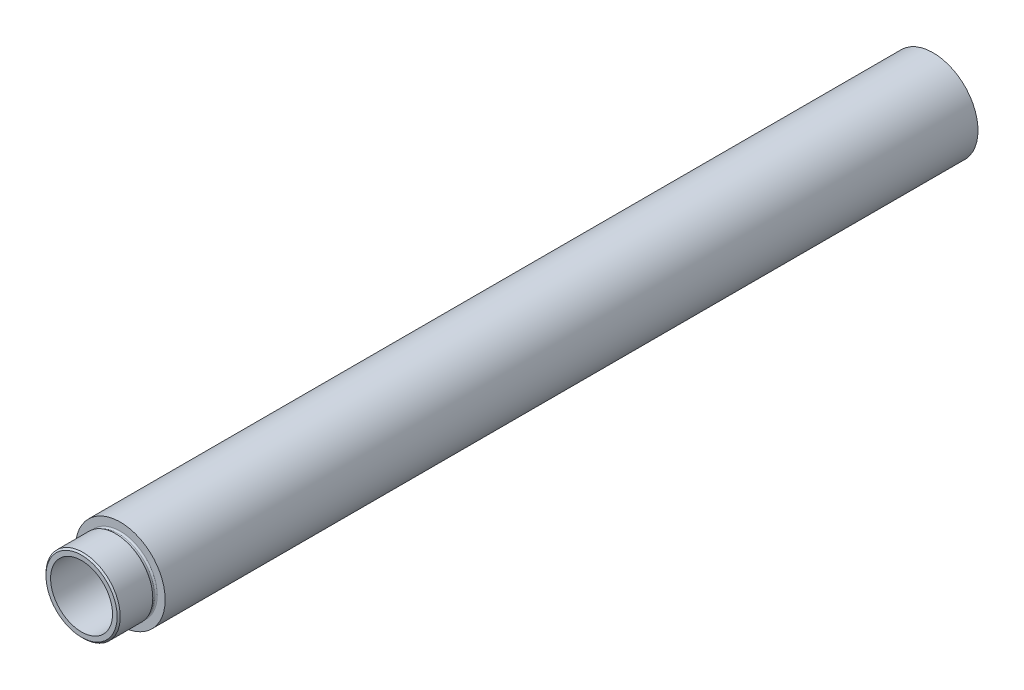
from build123d import *

# Parameters (mm, degrees)
SKETCH1_R           = 29
BOSS_EXTRUDE1_DEPTH = 550
CUT_EXTRUDE1_START  = -25
SKETCH2_R           = 29
SKETCH2_R_2         = 24
CUT_EXTRUDE1_DEPTH  = 25
SKETCH3_R           = 20
CUT_EXTRUDE2_DEPTH  = 552.526971235
CHAMFER1_SIZE       = 1
SKETCH4_R           = 24
SKETCH4_R_2         = 22.9
CUT_EXTRUDE3_DEPTH  = 3
FILLET1_R           = 1


with BuildPart() as part:
    # Sketch1 → Boss-Extrude1 (new body)
    with BuildSketch(Plane.XY):
        Circle(SKETCH1_R)
    extrude(amount=BOSS_EXTRUDE1_DEPTH)

    # Sketch2 → Cut-Extrude1 (cut)
    with BuildSketch(Plane.XY.offset(550).offset(CUT_EXTRUDE1_START)):
        Circle(SKETCH2_R)
        Circle(SKETCH2_R_2, mode=Mode.SUBTRACT)
    extrude(amount=CUT_EXTRUDE1_DEPTH, mode=Mode.SUBTRACT)

    # Sketch3 → Cut-Extrude2 (cut, through all)
    with BuildSketch(Plane.XY.offset(550)):
        Circle(SKETCH3_R)
    extrude(amount=-CUT_EXTRUDE2_DEPTH, mode=Mode.SUBTRACT)

    # Chamfer1
    chamfer1_edges = [part.edges().sort_by_distance(p)[0] for p in [
        (-24, 0, 550),
    ]]
    chamfer(chamfer1_edges, length=CHAMFER1_SIZE)

    # Sketch4 → Cut-Extrude3 (cut)
    with BuildSketch(Plane.XY.offset(525)):
        Circle(SKETCH4_R)
        Circle(SKETCH4_R_2, mode=Mode.SUBTRACT)
    extrude(amount=CUT_EXTRUDE3_DEPTH, mode=Mode.SUBTRACT)

    # Fillet1
    fillet1_edges = [part.edges().sort_by_distance(p)[0] for p in [
        (-22.9, 0, 525),
        (-22.9, 0, 528),
    ]]
    fillet(fillet1_edges, radius=FILLET1_R)


solid = part.part
